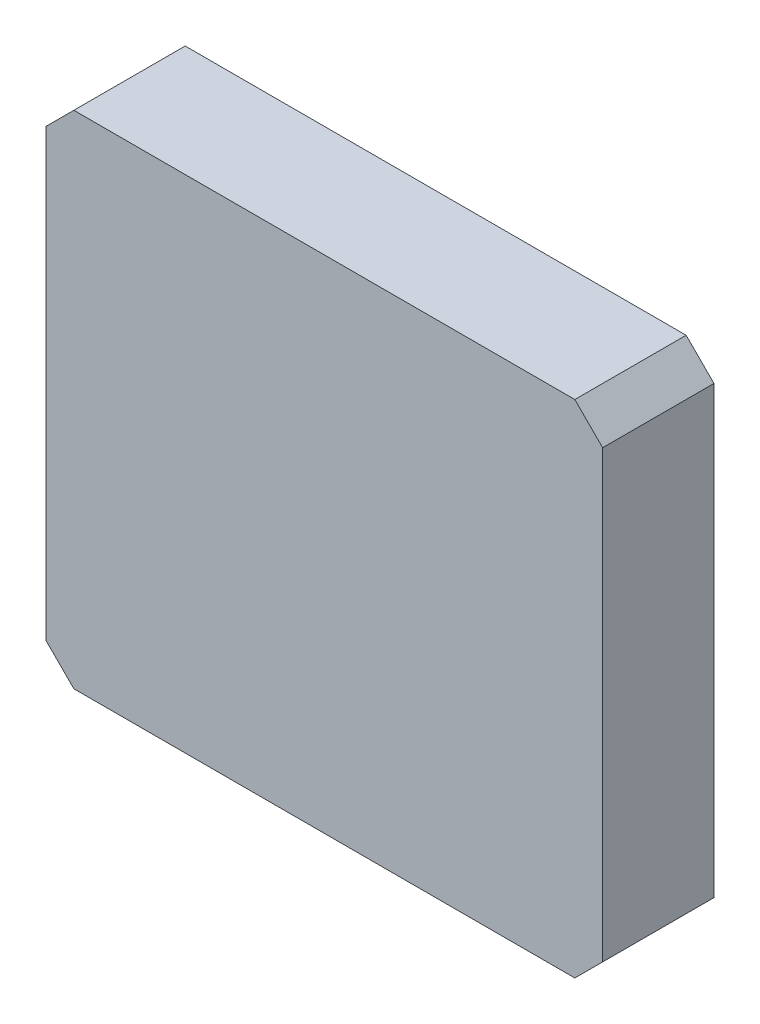
from build123d import *

# Parameters (mm, degrees)
SKETCH1_W           = 100
SKETCH1_H           = 90
BOSS_EXTRUDE1_DEPTH = 20
CHAMFER1_SIZE       = 5


with BuildPart() as part:
    # Sketch1 → Boss-Extrude1 (new body)
    with BuildSketch(Plane.XY):
        with Locations((3.384206163, 2.258064516)):
            Rectangle(SKETCH1_W, SKETCH1_H)
    extrude(amount=BOSS_EXTRUDE1_DEPTH)

    # Chamfer1
    chamfer1_edges = [part.edges().sort_by_distance(p)[0] for p in [
        (-46.615793837, 47.258064516, 10),
        (53.384206163, 47.258064516, 10),
        (53.384206163, -42.741935484, 10),
        (-46.615793837, -42.741935484, 10),
    ]]
    chamfer(chamfer1_edges, length=CHAMFER1_SIZE)


solid = part.part
